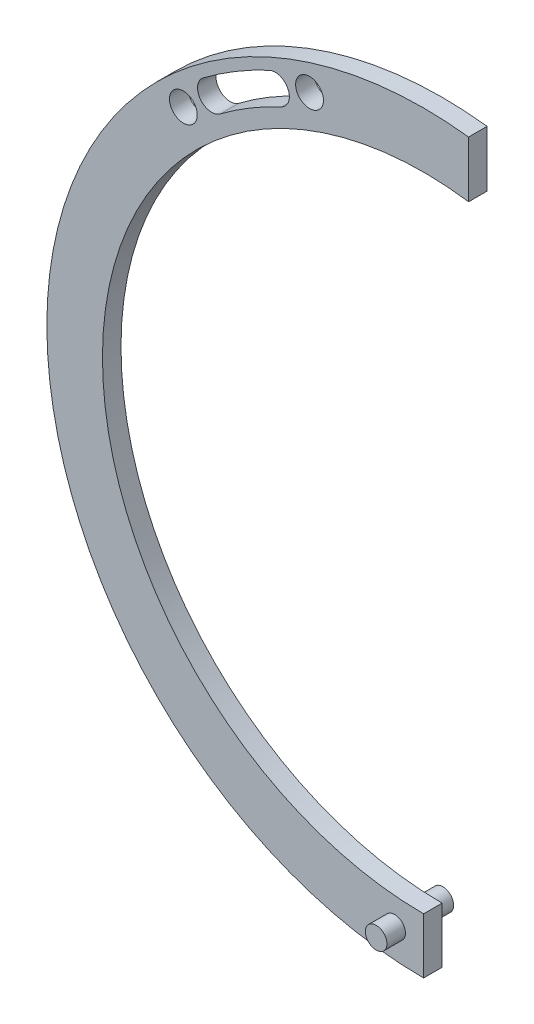
from build123d import *

# Parameters (mm, degrees)
BOSS_EXTRUDE1_DEPTH      = 10
BOSS_EXTRUDE2_DEPTH      = 10
BOSS_EXTRUDE2_DEPTH_BACK = 26
SKETCH2_R                = 5.820264096
CUT_EXTRUDE4_DEPTH       = 628.950741751
CUT_EXTRUDE4_DEPTH_BACK  = 628.950741751
SKETCH7_R                = 7.5


with BuildPart() as part:
    # Sketch1 → Boss-Extrude1 (new body)
    with BuildSketch(Plane.XY):
        with BuildLine():
            Line((-267.317020812, 384.57192575), (-267.301609192, 354.315771574))
            ThreePointArc((-267.301609192, 354.315771574), (-464.45214838, 194.902560898), (-291.585214163, 9.435771703))
            Line((-291.585214163, 9.435771703), (-291.585214163, -20.564228297))
            ThreePointArc((-291.585214163, -20.564228297), (-494.516390011, 194.886544), (-267.317020812, 384.57192575))
        make_face()
    extrude(amount=-BOSS_EXTRUDE1_DEPTH)

    # Sketch2 → Boss-Extrude2 (add, two sides: drawn at the far end of the back side and taken through both)
    with BuildSketch(Plane.XY.offset(-BOSS_EXTRUDE2_DEPTH_BACK)):
        with Locations((-307.201523558, -4.519874966)):
            Circle(SKETCH2_R)
    extrude(amount=BOSS_EXTRUDE2_DEPTH + BOSS_EXTRUDE2_DEPTH_BACK)

    # Sketch7 → Cut-Extrude4 (cut, two sides: drawn at the far end of the back side and taken through both)
    with BuildSketch(Plane(origin=(0, 0, -10), x_dir=(-1, 0, 0), z_dir=(0, 0, -1)).offset(-CUT_EXTRUDE4_DEPTH_BACK)):
        with Locations((421.223956701, 321.632808197)):
            Circle(SKETCH7_R)
        with Locations((353.128945359, 362.487113382)):
            Circle(SKETCH7_R)
        with BuildLine():
            ThreePointArc((410.530018999, 340.598670168), (393.284643136, 352.222259331), (374.913443912, 361.969559097))
            ThreePointArc((374.913443912, 361.969559097), (364.73585061, 358.251882975), (368.453526733, 348.074289673))
            ThreePointArc((368.453526733, 348.074289673), (385.400521629, 339.082637175), (401.308971217, 328.360152279))
            ThreePointArc((401.308971217, 328.360152279), (412.038754052, 329.868887332), (410.530018999, 340.598670168))
        make_face()
    extrude(amount=CUT_EXTRUDE4_DEPTH + CUT_EXTRUDE4_DEPTH_BACK, mode=Mode.SUBTRACT)


solid = part.part
